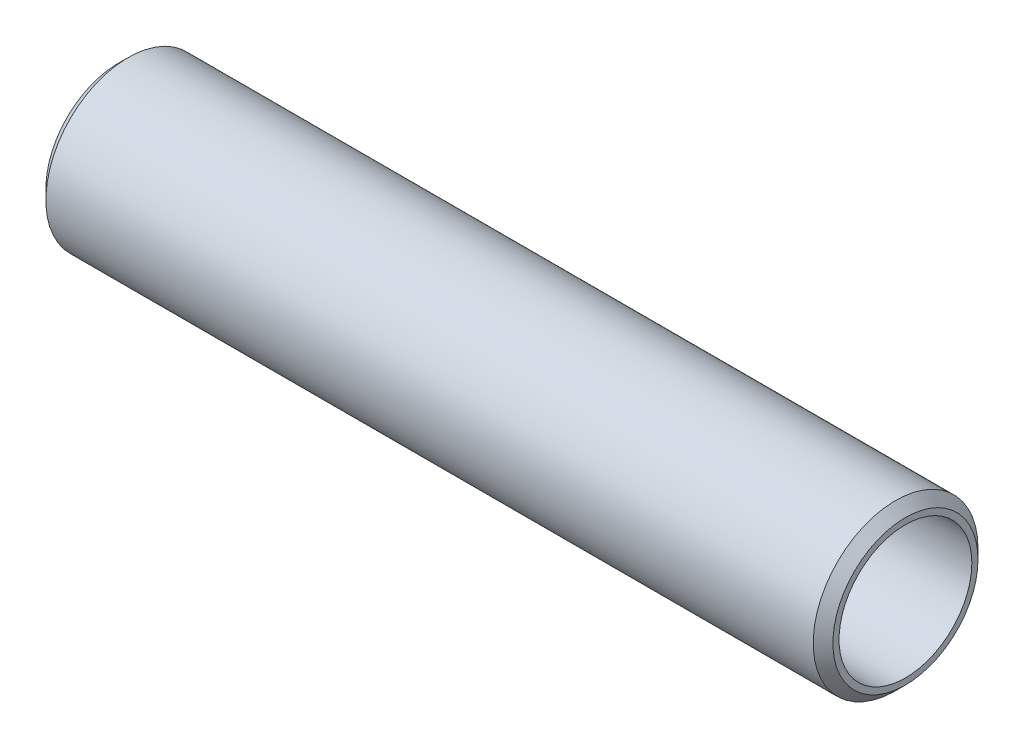
SolidWorks part; units mm, degrees
material "镀锌焊接钢管 Q215A"
ref_plane "前视基准面" through (0, 0, 0) normal (0, 0, 1) x (1, 0, 0)
ref_plane "上视基准面" through (0, 0, 0) normal (0, 1, 0) x (1, 0, 0)
ref_plane "右视基准面" through (0, 0, 0) normal (1, 0, 0) x (0, 0, -1)
sketch "草图1" plane through (0, 0, 0) normal (1, 0, 0) x (0, 0, -1)
  circle A0 centre (0, 0) radius 16.75
  dimension "D1" = 33.5
extrude "拉伸-薄壁1" add sketch "草图1" along normal blind 160 thin thin type one direction reverse wall 3.25
cosmetic thread "装饰螺纹线1" parameters "D1"=20, "D2"=30.291
cosmetic thread "装饰螺纹线2" parameters "D1"=20, "D2"=30.291
chamfer "倒角1" distance 2 angle 45 2 edges at (160, 0, -16.75) (0, 0, -16.75)
